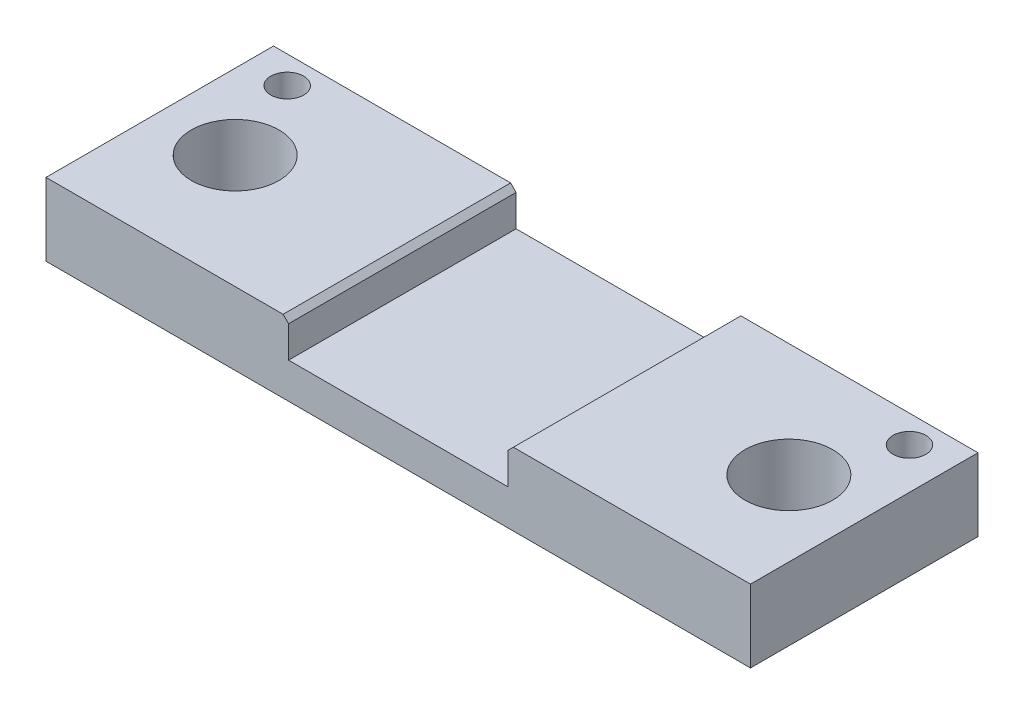
SolidWorks part; units mm, degrees
ref_plane "Front Plane" through (0, 0, 0) normal (0, 0, 1) x (1, 0, 0)
ref_plane "Top Plane" through (0, 0, 0) normal (0, 1, 0) x (1, 0, 0)
ref_plane "Right Plane" through (0, 0, 0) normal (1, 0, 0) x (0, 0, -1)
sketch "Sketch1" plane through (0, 0, 0) normal (0, 1, 0) x (1, 0, 0)
  line L0 (0, 0) -> (0, -50000) construction
  line L1 (-12.85, 4.15) -> (12.85, 4.15)
  line L2 (-12.85, 4.15) -> (-12.85, -4.15)
  line L3 (-12.85, -4.15) -> (12.85, -4.15)
  line L4 (12.85, 4.15) -> (12.85, -4.15)
  line L5 (-12.85, 4.15) -> (12.85, -4.15) construction
  line L6 (-12.85, -4.15) -> (12.85, 4.15) construction
  circle A0 centre (-10.1, 0) radius 1.6
  circle A1 centre (-11.35, 3.15) radius 0.6
  circle A2 centre (11.35, 3.15) radius 0.6
  circle A3 centre (10.1, 0) radius 1.6
  point P0 (0, 0)
  dimension "D7" = 3.2
  dimension "D8" = 1.2
  dimension "D1" = 25.7
  dimension "D2" = 8.3
  dimension "D3" = 20.2
  dimension "D4" = 22.7
  dimension "D5" = 1
extrude "Boss-Extrude1" add sketch "Sketch1" along normal blind 2.65
sketch "Sketch2" plane through (0, 2.65, 0) normal (0, 1, 0) x (1, 0, 0)
  line L0 (-12.85, -4.15) -> (12.85, -4.15) construction
  line L1 (-4, 4.15) -> (4, 4.15)
  line L2 (-4, 4.15) -> (-4, -4.15)
  line L3 (-4, -4.15) -> (4, -4.15)
  line L4 (4, 4.15) -> (4, -4.15)
  line L5 (-4, 4.15) -> (4, -4.15) construction
  line L6 (-4, -4.15) -> (4, 4.15) construction
  point P0 (0, 0)
  dimension "D1" = 8
extrude "Cut-Extrude1" cut sketch "Sketch2" against normal blind 1.35
chamfer "Chamfer1" distance 0.2 angle 45 2 edges at (4, 2.65, 0) (-4, 2.65, 0)
